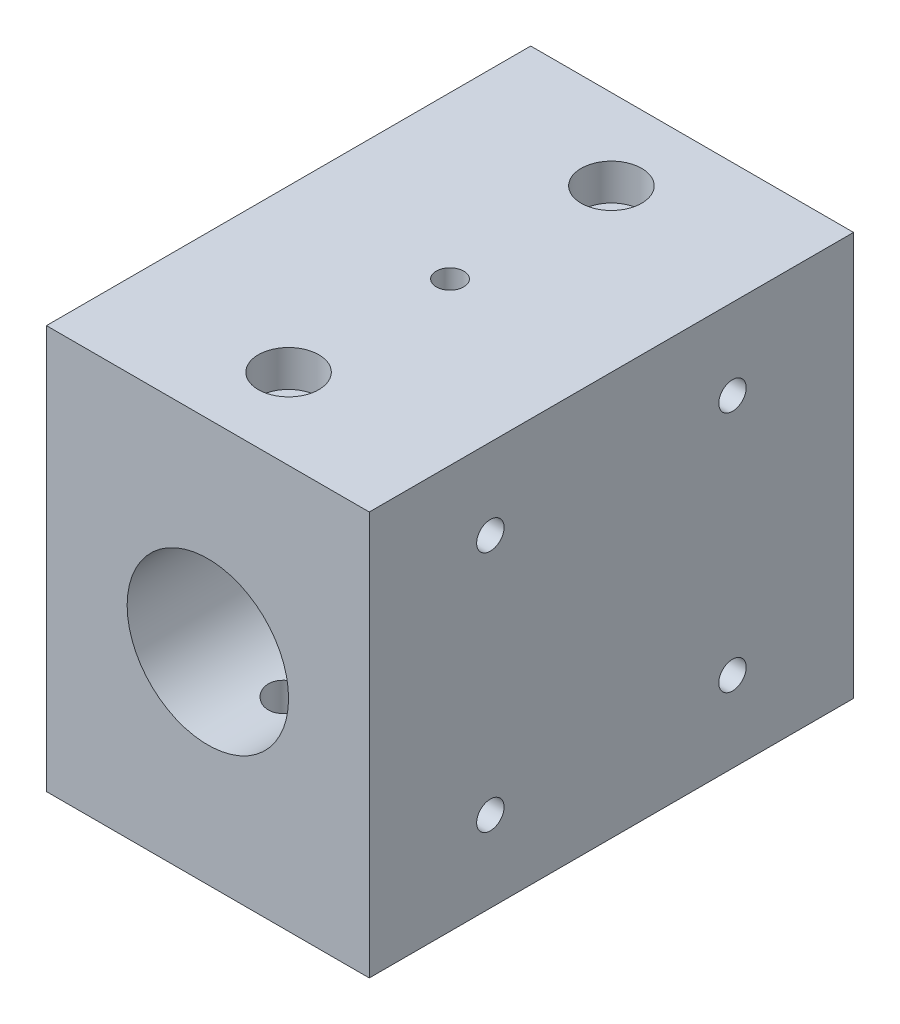
from build123d import *

# Parameters (mm, degrees)
SKETCH1_W                                          = 80
SKETCH1_H                                          = 100
BOSS_EXTRUDE1_DEPTH                                = 120
SKETCH2_R                                          = 20
CUT_EXTRUDE1_DEPTH                                 = 137.014705087
HOLE_SIZE_BASED_ON_HEX_SOCKET_CAP_SCRE_D           = 10
HOLE_SIZE_BASED_ON_HEX_SOCKET_CAP_SCRE_DEPTH       = 35
HOLE_SIZE_BASED_ON_HEX_SOCKET_CAP_SCRE_CBORE_D     = 15
HOLE_SIZE_BASED_ON_HEX_SOCKET_CAP_SCRE_CBORE_DEPTH = 9
HOLE_SIZE_BASED_ON_HEX_SOCKET_CAP_SCRE_TIP         = 3.004303095
HOLE_WIZARD_2_D                                    = 10
HOLE_WIZARD_2_DEPTH                                = 50
HOLE_WIZARD_2_CBORE_D                              = 15
HOLE_WIZARD_2_CBORE_DEPTH                          = 9
HOLE_WIZARD_2_TIP                                  = 3.004303095
M8_TAPPED_HOLE1_D                                  = 6.8
M8_TAPPED_HOLE1_DEPTH                              = 30
M8_TAPPED_HOLE1_TIP                                = 2.042926105
M8_TAPPED_HOLE2_D                                  = 6.8
M8_TAPPED_HOLE2_DEPTH                              = 30
M8_TAPPED_HOLE2_TIP                                = 2.042926105
M8_TAPPED_HOLE3_D                                  = 6.8
M8_TAPPED_HOLE3_DEPTH                              = 45
M8_TAPPED_HOLE3_TIP                                = 2.042926105


with BuildPart() as part:
    # Sketch1 → Boss-Extrude1 (new body)
    with BuildSketch(Plane.XY):
        Rectangle(SKETCH1_W, SKETCH1_H)
    extrude(amount=BOSS_EXTRUDE1_DEPTH)

    # Sketch2 → Cut-Extrude1 (cut, through all)
    with BuildSketch(Plane.XY.offset(120)):
        Circle(SKETCH2_R)
    extrude(amount=-CUT_EXTRUDE1_DEPTH, mode=Mode.SUBTRACT)

    # Hole Size (based on) hex socket cap screw type 2
    with Locations(Plane(origin=(0, 50, 0), x_dir=(1, 0, 0), z_dir=(0, 1, 0))):
        with Locations((0, -20), (0, -100)):
            CounterBoreHole(HOLE_SIZE_BASED_ON_HEX_SOCKET_CAP_SCRE_D / 2, HOLE_SIZE_BASED_ON_HEX_SOCKET_CAP_SCRE_CBORE_D / 2, HOLE_SIZE_BASED_ON_HEX_SOCKET_CAP_SCRE_CBORE_DEPTH, depth=HOLE_SIZE_BASED_ON_HEX_SOCKET_CAP_SCRE_DEPTH)
            with Locations((0, 0, -(HOLE_SIZE_BASED_ON_HEX_SOCKET_CAP_SCRE_DEPTH + HOLE_SIZE_BASED_ON_HEX_SOCKET_CAP_SCRE_TIP / 2))):  # 118° drill point
                Cone(0, HOLE_SIZE_BASED_ON_HEX_SOCKET_CAP_SCRE_D / 2, HOLE_SIZE_BASED_ON_HEX_SOCKET_CAP_SCRE_TIP, mode=Mode.SUBTRACT)

    # 打孔尺寸(%根据)内六角圆柱头螺钉的类型2
    with Locations(Plane(origin=(0, -50, 0), x_dir=(-1, 0, 0), z_dir=(0, -1, 0))):
        with Locations((0, -20), (0, -100)):
            CounterBoreHole(HOLE_WIZARD_2_D / 2, HOLE_WIZARD_2_CBORE_D / 2, HOLE_WIZARD_2_CBORE_DEPTH, depth=HOLE_WIZARD_2_DEPTH)
            with Locations((0, 0, -(HOLE_WIZARD_2_DEPTH + HOLE_WIZARD_2_TIP / 2))):  # 118° drill point
                Cone(0, HOLE_WIZARD_2_D / 2, HOLE_WIZARD_2_TIP, mode=Mode.SUBTRACT)

    # M8 Tapped Hole1
    with Locations(Plane.ZY.offset(40)):
        with Locations((30, 30), (90, 30), (90, -30), (30, -30)):
            Hole(M8_TAPPED_HOLE1_D / 2, depth=M8_TAPPED_HOLE1_DEPTH)
            with Locations((0, 0, -(M8_TAPPED_HOLE1_DEPTH + M8_TAPPED_HOLE1_TIP / 2))):  # 118° drill point
                Cone(0, M8_TAPPED_HOLE1_D / 2, M8_TAPPED_HOLE1_TIP, mode=Mode.SUBTRACT)

    # M8 Tapped Hole2
    with Locations(Plane(origin=(40, 0, 0), x_dir=(0, 0, -1), z_dir=(1, 0, 0))):
        with Locations((-90, 30), (-30, 30), (-30, -30), (-90, -30)):
            Hole(M8_TAPPED_HOLE2_D / 2, depth=M8_TAPPED_HOLE2_DEPTH)
            with Locations((0, 0, -(M8_TAPPED_HOLE2_DEPTH + M8_TAPPED_HOLE2_TIP / 2))):  # 118° drill point
                Cone(0, M8_TAPPED_HOLE2_D / 2, M8_TAPPED_HOLE2_TIP, mode=Mode.SUBTRACT)

    # M8 Tapped Hole3
    with Locations(Plane(origin=(0, 50, 0), x_dir=(1, 0, 0), z_dir=(0, 1, 0))):
        with Locations((0, -60)):
            Hole(M8_TAPPED_HOLE3_D / 2, depth=M8_TAPPED_HOLE3_DEPTH)
            with Locations((0, 0, -(M8_TAPPED_HOLE3_DEPTH + M8_TAPPED_HOLE3_TIP / 2))):  # 118° drill point
                Cone(0, M8_TAPPED_HOLE3_D / 2, M8_TAPPED_HOLE3_TIP, mode=Mode.SUBTRACT)


solid = part.part
